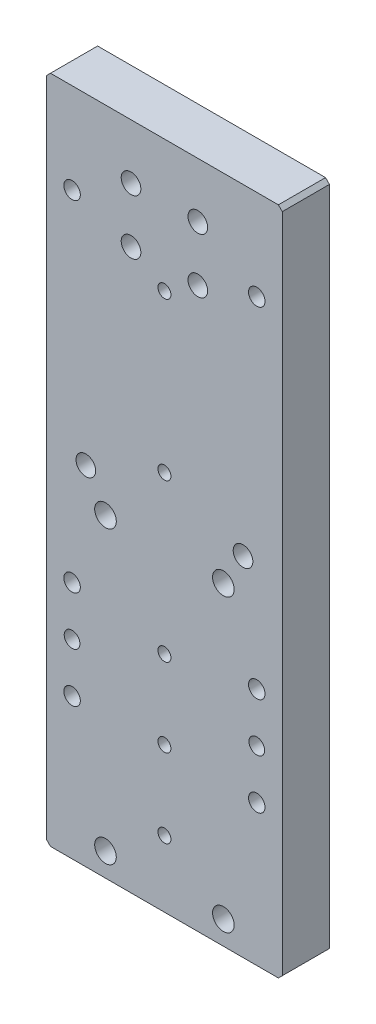
SolidWorks part; units mm, degrees
material "AL6061"
ref_plane "Front" through (0, 0, 0) normal (0, 0, 1) x (1, 0, 0)
ref_plane "Top" through (0, 0, 0) normal (0, 1, 0) x (1, 0, 0)
ref_plane "Right" through (0, 0, 0) normal (1, 0, 0) x (0, 0, -1)
sketch "Sketch1" plane through (0, 0, 0) normal (0, 0, 1) x (1, 0, 0)
  line L1 (-30, 85.2) -> (30, 85.2)
  line L2 (-30, 85.2) -> (-30, -85.2)
  line L3 (-30, -85.2) -> (30, -85.2)
  line L4 (30, 85.2) -> (30, -85.2)
  line L5 (-30, 85.2) -> (30, -85.2) construction
  line L6 (-30, -85.2) -> (30, 85.2) construction
  point P0 (0, 0)
  dimension "D1" = 170.4
  dimension "D2" = 60
extrude "Boss-Extrude1" add sketch "Sketch1" along normal mid plane 12
hole_wizard "CBORE for M5 Hex Socket Head Cap Screw1" positions "Sketch4" profile "Sketch5" counterbore size "M5" standard "ISO" end condition through all
sketch "Sketch4" plane through (0, 0, -6) normal (0, 0, -1) x (-1, 0, 0)
  point P0 (15, -5.2)
  point P3 (-15, -5.2)
  point P6 (15, -79.2)
  point P9 (-15, -79.2)
sketch "Sketch5" plane through (-15, -5.2, -6) normal (1, 0, 0) x (0, 1, 0)
  line L0 (0, 0) -> (0, 12)
  line L1 (0, 12) -> (2.75, 12)
  line L3 (2.75, 12) -> (2.75, 5.4)
  line L4 (2.75, 5.4) -> (5, 5.4)
  line L5 (5, 5.4) -> (5, 0)
  line L7 (5, 0) -> (0, 0)
  line L11 (0, -6.35) -> (0, 107.95) construction
  dimension "通孔孔直径" = 5.5
  dimension "通孔孔深度" = 12
  dimension "柱形沉头孔直径" = 10
  dimension "柱形沉头孔深度" = 5.4
hole_wizard "Blind pin hole0" positions "Sketch6" profile "Sketch7" hole size "Ø5.0" standard "ISO" end condition through all
sketch "Sketch6" plane through (0, 0, 6) normal (0, 0, 1) x (1, 0, 0)
  line L0 (-27, 0.8) -> (27, 0.8) construction
  line L1 (0, 0) -> (0, 19.9741) construction
  point P0 (20, 3.3)
  point P2 (-20, 3.3)
  dimension "D1" = 2.5
  dimension "D2" = 40
sketch "Sketch7" plane through (20, 3.3, 6) normal (1, 0, 0) x (0, -1, 0)
  line L0 (0, 0) -> (0, 12)
  line L1 (0, 12) -> (2.5, 12)
  line L2 (2.5, 12) -> (2.5, 0)
  line L5 (2.5, 0) -> (0, 0)
  line L11 (0, -6.35) -> (0, 107.95) construction
  dimension "通孔孔直径" = 5
  dimension "通孔孔深度" = 12
hole_wizard "M4 Tapped Hole1" positions "Sketch10" profile "Sketch9" tap size "M4" standard "ISO" end condition through all
sketch "Sketch10" plane through (0, 0, -6) normal (0, 0, -1) x (-1, 0, 0)
  point P0 (0, 11.7)
  point P3 (0, -28.3)
  point P6 (0, -48.3)
  point P9 (0, -68.3)
  point P13 (0, 51.7)
  dimension "D1" = 40
sketch "Sketch9" plane through (0, 11.7, -6) normal (1, 0, 0) x (0, 1, 0)
  line L0 (0, 0) -> (0, 12)
  line L1 (0, 12) -> (1.65, 12)
  line L2 (1.65, 12) -> (1.65, 0)
  line L5 (1.65, 0) -> (0, 0)
  line L11 (0, -6.35) -> (0, 107.95) construction
  dimension "通孔螺纹孔钻头直径" = 3.3
  dimension "通孔螺纹孔钻头深度" = 12
cosmetic thread "Cosmetic Thread2" parameters "D2"=4
cosmetic thread "Cosmetic Thread3" parameters "D2"=4
cosmetic thread "Cosmetic Thread4" parameters "D2"=4
cosmetic thread "Cosmetic Thread10" parameters "D2"=4
cosmetic thread "Cosmetic Thread11" parameters "D2"=4
sketch "Sketch11" plane through (0, 0, -6) normal (0, 0, -1) x (-1, 0, 0)
  circle A0 centre (0, 51.7) radius 3.5
  circle A1 centre (0, -68.3) radius 3.5
  dimension "D1" = 7
extrude "Cut-Extrude1" cut sketch "Sketch11" against normal blind 2
hole_wizard "M6 Tapped Hole1" positions "Sketch12" profile "Sketch13" tap size "M6" standard "ISO"
sketch "Sketch12" plane through (0, 0, 6) normal (0, 0, 1) x (1, 0, 0)
  line L0 (-6.5, 53.7) -> (-10.5, 53.7) construction
  line L2 (0, 0) -> (0, 34.9244) construction
  line L5 (-6.5, 67.7) -> (-10.5, 67.7) construction
  arc A0 (-10.5, 60.7) -> (-10.5, 53.7) centre (-10.5, 57.2) ccw construction
  point P0 (8.5, 57.2)
  point P2 (-8.5, 57.2)
  point P4 (8.5, 71.2)
  point P6 (-8.5, 71.2)
  dimension "D1" = 3.5
  dimension "D2" = 2
  dimension "D3" = 3.5
sketch "Sketch13" plane through (8.5, 57.2, 6) normal (1, 0, 0) x (0, -1, 0)
  line L0 (0, 0) -> (0, 18.5022)
  line L1 (0, 18.5022) -> (2.5, 17)
  line L2 (2.5, 17) -> (2.5, 0)
  line L5 (2.5, 0) -> (0, 0)
  line L10 (0, 18.5022) -> (-2.5, 17) construction
  line L11 (0, -6.35) -> (0, 107.95) construction
  dimension "螺纹孔钻头直径" = 5
  dimension "螺纹孔钻头深度" = 17
  dimension "导头角度" = 118
cosmetic thread "Cosmetic Thread6" parameters "D1"=12, "D2"=6
cosmetic thread "Cosmetic Thread7" parameters "D1"=12, "D2"=6
cosmetic thread "Cosmetic Thread8" parameters "D1"=12, "D2"=6
cosmetic thread "Cosmetic Thread9" parameters "D1"=12, "D2"=6
chamfer "Chamfer1" distance 1 angle 45 4 edges at (-30, -85.2, 0) (30, -85.2, 0) (30, 85.2, 0) (-30, 85.2, 0)
hole_wizard "Blind pin hole1" positions "Sketch14" profile "Sketch15" hole size "Ø4.0" standard "ISO" end condition through all
sketch "Sketch14" plane through (0, 0, -6) normal (0, 0, -1) x (-1, 0, 0)
  line L0 (0, 85.2) -> (0, -85.2) construction
  line L1 (-29, 85.2) -> (29, 85.2) construction
  line L2 (29, -85.2) -> (-29, -85.2) construction
  line L5 (-44.5168, -36.8) -> (35.3597, -36.8) construction
  line L6 (-30, -84.2) -> (-30, 84.2) construction
  point P16 (-23.5, -36.8)
  point P21 (23.5, -36.8)
  dimension "D1" = 48.4
  dimension "D2" = 6.5
sketch "Sketch15" plane through (-23.5, -36.8, -6) normal (1, 0, 0) x (0, 1, 0)
  line L0 (0, 0) -> (0, 12)
  line L1 (0, 12) -> (2, 12)
  line L2 (2, 12) -> (2, 0)
  line L5 (2, 0) -> (0, 0)
  line L11 (0, -6.35) -> (0, 107.95) construction
  dimension "通孔孔直径" = 4
  dimension "通孔孔深度" = 12
hole_wizard "M5 Tapped Hole1" positions "Sketch18" profile "Sketch19" tap size "M5" standard "ISO" end condition through all
sketch "Sketch18" plane through (0, 0, -6) normal (0, 0, -1) x (-1, 0, 0)
  line L0 (-23.5, -36.8) -> (23.5, -36.8) construction
  line L3 (0, -85.2) -> (0, -15.4653) construction
  line L4 (29, -85.2) -> (-29, -85.2) construction
  point P15 (-23.5, -24.3)
  point P18 (-23.5, -49.3)
  point P19 (23.5, -49.3)
  point P20 (23.5, -24.3)
  point P23 (-23.5, 62.2)
  point P26 (23.5, 62.2)
  dimension "D2" = 47
  dimension "D1" = 25
  dimension "D3" = 86.5
sketch "Sketch19" plane through (-23.5, 62.2, -6) normal (1, 0, 0) x (0, 1, 0)
  line L0 (0, 0) -> (0, 12)
  line L1 (0, 12) -> (2.1, 12)
  line L2 (2.1, 12) -> (2.1, 0)
  line L5 (2.1, 0) -> (0, 0)
  line L11 (0, -6.35) -> (0, 107.95) construction
  dimension "通孔螺纹孔钻头直径" = 4.2
  dimension "通孔螺纹孔钻头深度" = 12
cosmetic thread "Cosmetic Thread12" parameters "D2"=5
cosmetic thread "Cosmetic Thread13" parameters "D2"=5
cosmetic thread "Cosmetic Thread14" parameters "D2"=5
cosmetic thread "Cosmetic Thread15" parameters "D2"=5
cosmetic thread "Cosmetic Thread16" parameters "D2"=5
cosmetic thread "Cosmetic Thread17" parameters "D2"=5
